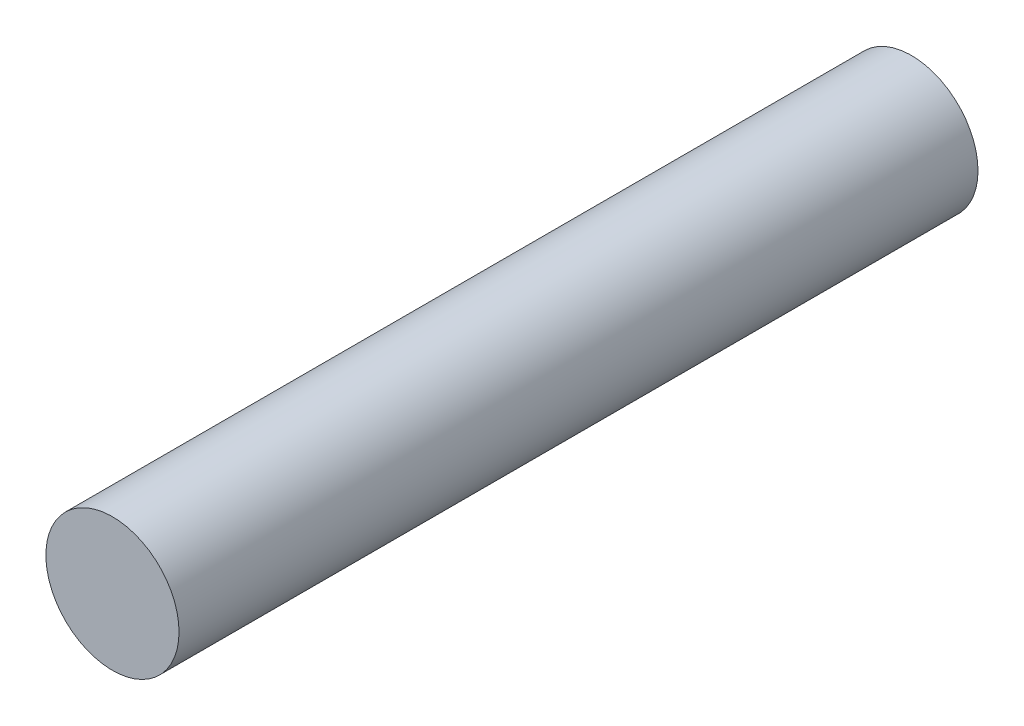
from build123d import *

# Parameters (mm, degrees)
SKETCH1_R           = 100
BOSS_EXTRUDE1_DEPTH = 1200


with BuildPart() as part:
    # Sketch1 → Boss-Extrude1 (new body)
    with BuildSketch(Plane.XY):
        Circle(SKETCH1_R)
    extrude(amount=BOSS_EXTRUDE1_DEPTH)


solid = part.part
